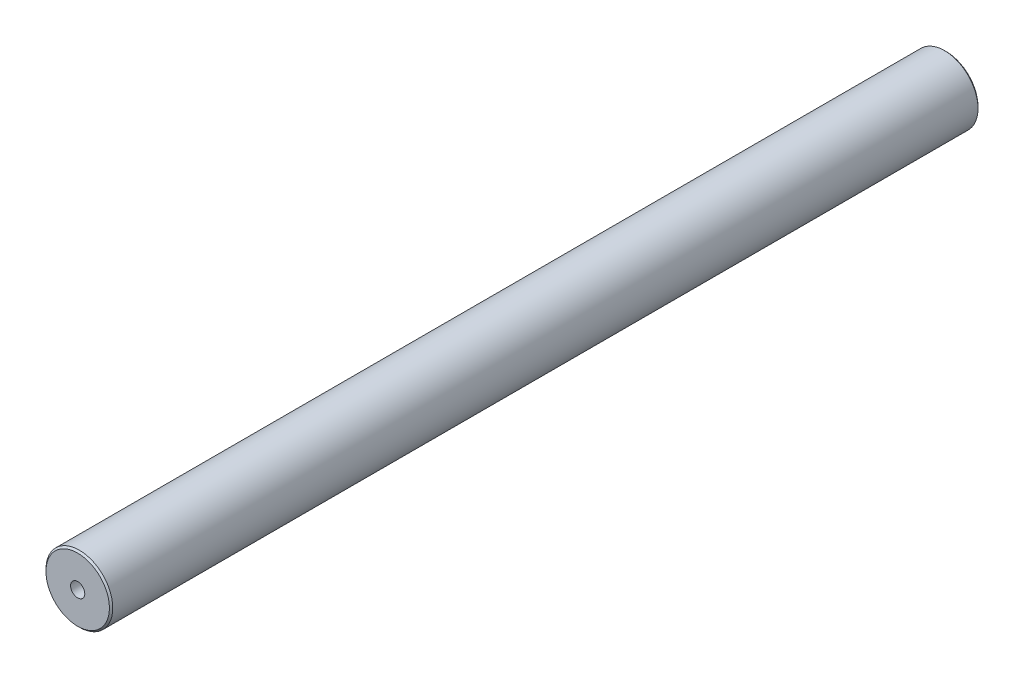
SolidWorks part; units mm, degrees
ref_plane "前视基准面" through (0, 0, 0) normal (0, 0, 1) x (1, 0, 0)
ref_plane "上视基准面" through (0, 0, 0) normal (0, 1, 0) x (1, 0, 0)
ref_plane "右视基准面" through (0, 0, 0) normal (1, 0, 0) x (0, 0, -1)
sketch "草图1" plane through (0, 0, 0) normal (0, 0, 1) x (1, 0, 0)
  circle A0 centre (0, 0) radius 20
  dimension "D1" = 40
extrude "凸台-拉伸1" add sketch "草图1" along normal blind 520 contours A0
hole_wizard "M10 螺纹孔1" positions "草图3" profile "草图4" tap size "M10" standard "ISO"
sketch "草图3" plane through (0, 0, 0) normal (0, 0, -1) x (-1, 0, 0)
  point P0 (0, 0)
sketch "草图4" plane through (0, 0, 0) normal (1, 0, 0) x (0, 1, 0)
  line L0 (0, 0) -> (0, 34.5537)
  line L1 (0, 34.5537) -> (4.25, 32)
  line L2 (4.25, 32) -> (4.25, 0)
  line L5 (4.25, 0) -> (0, 0)
  line L10 (0, 34.5537) -> (-4.25, 32) construction
  line L11 (0, -6.35) -> (0, 107.95) construction
  dimension "螺纹孔钻头直径" = 8.5
  dimension "螺纹孔钻头深度" = 32
  dimension "导头角度" = 118
cosmetic thread "孔螺蚊线1"
chamfer "倒角1" distance 1 angle 45 1 edges at (20, 0, 520)
chamfer "倒角2" distance 1 angle 45 1 edges at (20, 0, 0)
hole_wizard "M10 螺纹孔2" positions "草图6" profile "草图5" tap size "M10" standard "ISO"
sketch "草图6" plane through (0, 0, 520) normal (0, 0, 1) x (1, 0, 0)
  point P3 (0, 0)
sketch "草图5" plane through (0, 0, 520) normal (1, 0, 0) x (0, -1, 0)
  line L0 (0, 0) -> (0, 27.0537)
  line L1 (0, 27.0537) -> (4.25, 24.5)
  line L2 (4.25, 24.5) -> (4.25, 0)
  line L5 (4.25, 0) -> (0, 0)
  line L10 (0, 27.0537) -> (-4.25, 24.5) construction
  line L11 (0, -6.35) -> (0, 107.95) construction
  dimension "螺纹孔钻头直径" = 8.5
  dimension "螺纹孔钻头深度" = 24.5
  dimension "导头角度" = 118
cosmetic thread "孔螺蚊线2" parameters "D1"=20, "D2"=10
